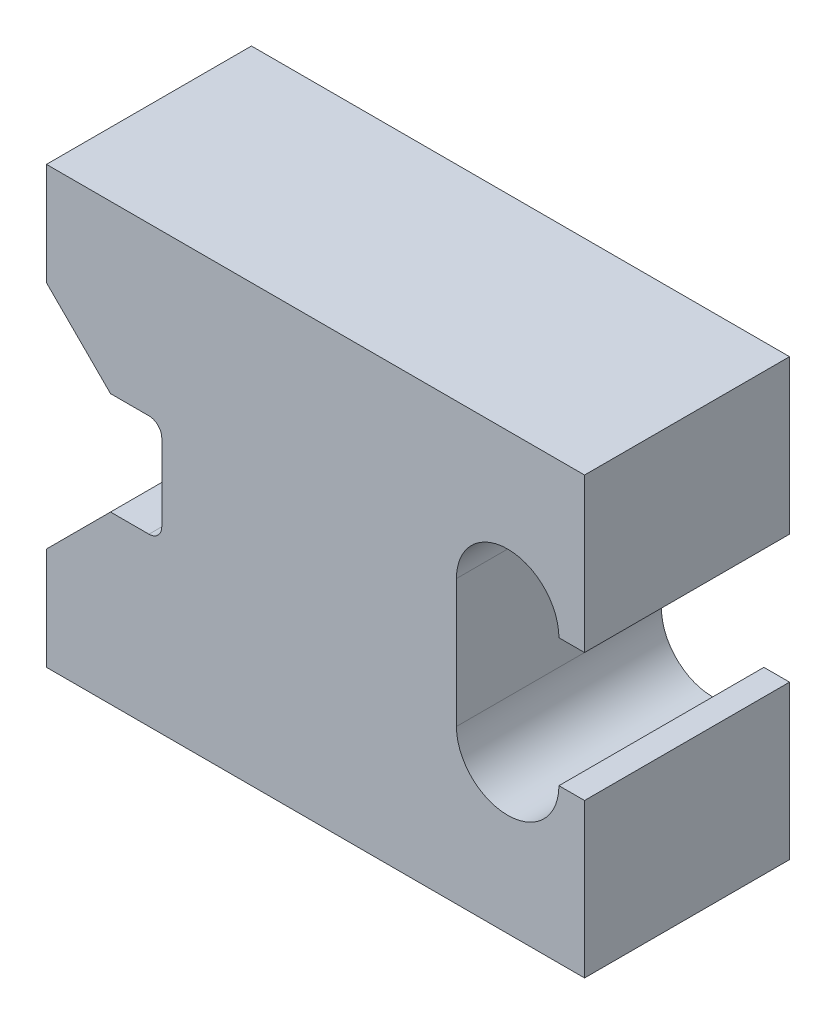
SolidWorks part; units mm, degrees
extrude "Base-Extrude" add sketch "Sketch1" along normal blind 16
sketch "Sketch1" plane through (0, 0, 0) normal (0, 0, 1) x (1, 0, 0)
  line L0 (-100, 0) -> (100, 0) construction
  line L1 (60, 17) -> (60, -17)
  line L2 (60, -17) -> (15, -17)
  line L3 (15, -17) -> (15, 17)
  line L4 (15, 17) -> (60, 17)
  point P7 (60, 0)
material "镍"
ref_plane "Front view" through (0, 0, 0) normal (0, 0, 1) x (1, 0, 0)
ref_plane "Top view" through (0, 0, 0) normal (0, 1, 0) x (1, 0, 0)
ref_plane "Right view" through (0, 0, 0) normal (1, 0, 0) x (0, 0, -1)
sketch "Sketch2" plane through (0, 0, 16) normal (0, 0, 1) x (1, 0, 0)
  line L0 (-50, 0) -> (60, 0) construction
  line L1 (27, 4) -> (27, -4)
  line L2 (15, 17) -> (15, -17) construction
  line L3 (15, 12) -> (15, -12)
  line L4 (27, -4) -> (23, -4)
  line L5 (27, 4) -> (23, 4)
  line L6 (23, 4) -> (15, 12)
  line L7 (23, -4) -> (15, -12)
  point P9 (15, 0)
extrude "Cut-Extrude1" cut sketch "Sketch2" against normal through all
fillet "Fillet1" radius 1 1 edges at (27, 4, 8)
fillet "Fillet2" radius 1 1 edges at (27, -4, 8)
sketch "Sketch4" plane through (0, 0, 16) normal (0, 0, 1) x (1, 0, 0)
  line L0 (-50, 0) -> (60, 0) construction
  line L1 (50, 5) -> (50, -5)
  line L2 (60, -17) -> (60, 17) construction
  line L3 (60, 5) -> (60, -5)
  line L4 (58, 5) -> (60, 5)
  line L6 (58, -5) -> (60, -5)
  arc A0 (50, -5) -> (58, -5) centre (54, -5) ccw
  arc A1 (50, 5) -> (58, 5) centre (54, 5) cw
extrude "Cut-Extrude3" cut sketch "Sketch4" against normal through all
sketch "Sketch5" plane through (0, 0, 16) normal (0, 0, 1) x (1, 0, 0)
  line L0 (15, 17) -> (18, 17)
  line L1 (60, 17) -> (15, 17) construction
  line L2 (18, 17) -> (18, -17)
  line L3 (15, -17) -> (60, -17) construction
  line L4 (18, -17) -> (15, -17)
  line L5 (15, -17) -> (15, 17)
extrude "Cut-Extrude4" cut sketch "Sketch5" against normal through all
equation "\"B/2@Sketch1\" = \"B@Sketch1\" / 2"
equation "\"D3@Sketch2\" = \"b4@Sketch2\" / 2"
equation "\"N/2@Sketch2\" = \"N@Sketch2\" / 2"
equation "\"D2@Sketch2\" = \"D1@Sketch2\""
equation "\"D1@Fillet1\" = \"r@Fillet2\""
equation "\"D5@Sketch4\" = \"b1@Sketch4\" / 2"
equation "\"D4@Sketch4\" = \"D1@Sketch4\""
equation "\"D2@Sketch4\" = \"D3@Sketch4\" * 2"
